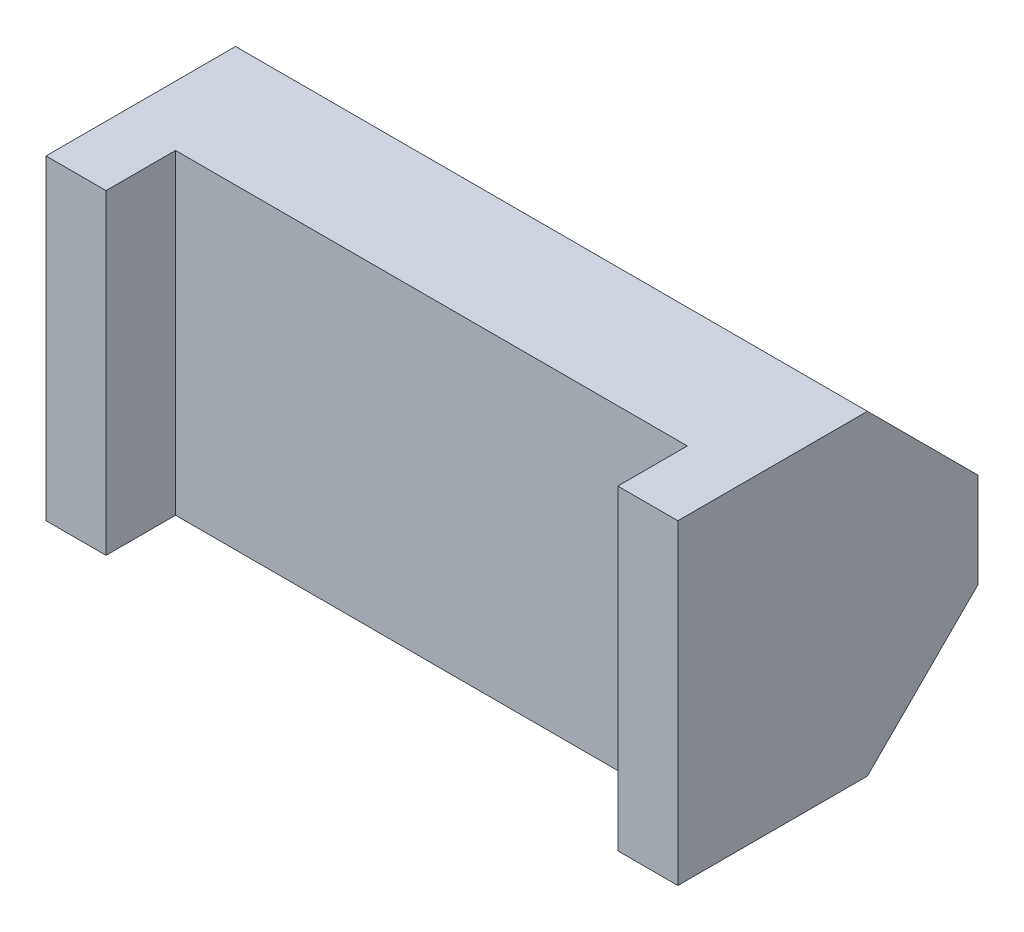
SolidWorks part; units mm, degrees
ref_plane "前视基准面" through (0, 0, 0) normal (0, 0, 1) x (1, 0, 0)
ref_plane "上视基准面" through (0, 0, 0) normal (0, 1, 0) x (1, 0, 0)
ref_plane "右视基准面" through (0, 0, 0) normal (1, 0, 0) x (0, 0, -1)
sketch "草图1" plane through (0, 0, 0) normal (0, 0, 1) x (1, 0, 0)
  line L0 (0, 5) -> (0, 0) construction
  line L1 (-10, 5) -> (10, 5)
  line L2 (-10, 5) -> (-10, -5)
  line L3 (-10, -5) -> (10, -5)
  line L4 (10, 5) -> (10, -5)
  line L5 (0, 0) -> (10, 0) construction
  dimension "D1" = 20
  dimension "D2" = 10
extrude "凸台-拉伸1" add sketch "草图1" along normal blind 9.5
sketch "草图2" plane through (0, 0, 9.5) normal (0, 0, 1) x (1, 0, 0)
  line L0 (0, 4.3603) -> (0, 0) construction
  line L1 (-8.1, 14.9476) -> (8.1, 14.9476)
  line L2 (-8.1, 14.9476) -> (-8.1, -14.9476)
  line L3 (-8.1, -14.9476) -> (8.1, -14.9476)
  line L4 (8.1, 14.9476) -> (8.1, -14.9476)
  line L5 (0, 0) -> (16.2, 0) construction
  dimension "D1" = 16.2
extrude "切除-拉伸1" cut sketch "草图2" against normal blind 2.2
sketch "草图3" plane through (-10, 0, 0) normal (-1, 0, 0) x (0, 0, 1)
  line L0 (0, 5) -> (3.5, 5)
  line L1 (9.5, 5) -> (0, 5) construction
  line L2 (3.5, 5) -> (0, 1.5)
  line L3 (0, 5) -> (0, -5) construction
  line L4 (0, 1.5) -> (0, 5)
  line L5 (0, 0) -> (3.2793, 0) construction
  dimension "D1" = 1.5
  dimension "D2" = 45
extrude "切除-拉伸2" cut sketch "草图3" against normal through all
mirror "镜向1" about plane through (0, 0, 0) normal (0, 1, 0) of "切除-拉伸2"
sketch "草图4" plane through (0, 0, 7.3) normal (0, 0, 1) x (1, 0, 0)
  circle A0 centre (0, 0) radius 1.9077
